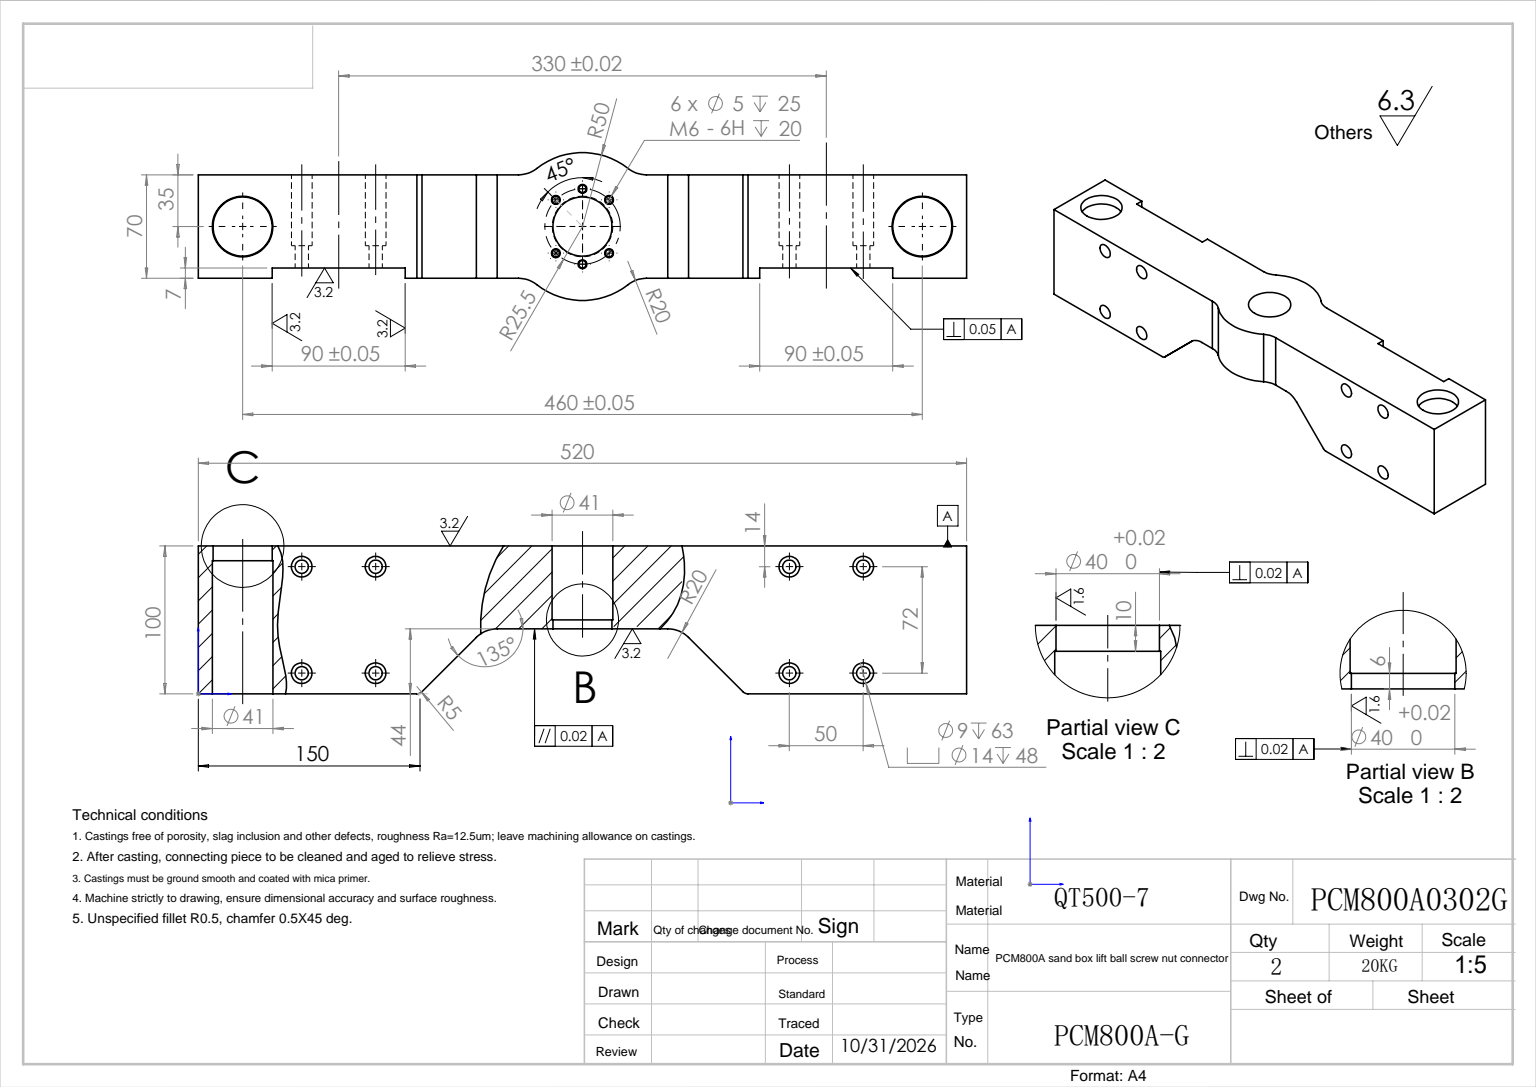
from build123d import *

# Parameters (mm, degrees)
EXTRUDE_1_DEPTH              = 100
CUT_EXTRUDE_1_DEPTH          = 537.306815172
CUT_EXTRUDE_1_DEPTH_BACK     = 537.306815172
SKETCH_3_R                   = 20
CUT_EXTRUDE_2_DEPTH          = 530.868882144
SKETCH_7_R                   = 4.5
CUT_EXTRUDE_4_DEPTH          = 536.242001341
SKETCH_8_R                   = 7
CUT_EXTRUDE_5_DEPTH          = 48
SKETCH_13_R                  = 20
CUT_EXTRUDE_7_DEPTH          = 537.306815172
SKETCH_12_R                  = 1
CUT_EXTRUDE_8_DEPTH          = 10
HOLE_WIZARD_M6_1_D           = 5
HOLE_WIZARD_M6_1_DEPTH       = 25
HOLE_WIZARD_M6_1_CBORE_D     = 6
HOLE_WIZARD_M6_1_CBORE_DEPTH = 20
HOLE_WIZARD_M6_1_TIP         = 1.502151548
SKETCH_18_R                  = 20.5
CUT_EXTRUDE_9_DEPTH          = 90
SKETCH_19_R                  = 20.5
CUT_EXTRUDE_10_DEPTH         = 50
FILLET_1_R                   = 5


with BuildPart() as part:
    # 草图1 → 拉伸1 (new body)
    with BuildSketch(Plane(origin=(0, 0, 0), x_dir=(1, 0, 0), z_dir=(0, 1, 0))):
        with BuildLine():
            Line((0, 70), (0, 0))
            Line((0, 0), (216.698729811, 0))
            ThreePointArc((216.698729811, 0), (223.245266518, -1.10177635), (229.070521293, -4.285714286))
            ThreePointArc((229.070521293, -4.285714286), (260, -15), (290.929478707, -4.285714286))
            ThreePointArc((290.929478707, -4.285714286), (296.754733482, -1.10177635), (303.301270189, 0))
            Line((303.301270189, 0), (520, 0))
            Line((520, 0), (520, 70))
            Line((520, 70), (470, 70))
            Line((470, 70), (470, 63))
            Line((470, 63), (380, 63))
            Line((380, 63), (380, 70))
            Line((380, 70), (303.301270189, 70))
            ThreePointArc((303.301270189, 70), (296.754733482, 71.10177635), (290.929478707, 74.285714286))
            ThreePointArc((290.929478707, 74.285714286), (260, 85), (229.070521293, 74.285714286))
            ThreePointArc((229.070521293, 74.285714286), (223.245266518, 71.10177635), (216.698729811, 70))
            Line((216.698729811, 70), (140, 70))
            Line((140, 70), (140, 63))
            Line((140, 63), (50, 63))
            Line((50, 63), (50, 70))
            Line((50, 70), (0, 70))
        make_face()
    extrude(amount=EXTRUDE_1_DEPTH)

    # 草图2 → 切除-拉伸1 (cut, two sides: drawn at the far end of the back side and taken through both)
    with BuildSketch(Plane.XY.offset(-CUT_EXTRUDE_1_DEPTH_BACK)):
        with BuildLine():
            Line((317.715767105, 43.999711923), (202.284232895, 43.999711923))
            ThreePointArc((202.284232895, 43.999711923), (194.630594492, 42.477315101), (188.142143567, 38.141893843))
            Line((188.142143567, 38.141893843), (150, 0))
            Line((150, 0), (370, 0))
            Line((370, 0), (331.857856433, 38.141893843))
            ThreePointArc((331.857856433, 38.141893843), (325.369405508, 42.477315101), (317.715767105, 43.999711923))
        make_face()
    extrude(amount=CUT_EXTRUDE_1_DEPTH + CUT_EXTRUDE_1_DEPTH_BACK, mode=Mode.SUBTRACT)

    # 草图3 → 切除-拉伸2 (cut, through all)
    with BuildSketch(Plane.XZ.offset(-43.999711923)):
        with Locations((260, -35)):
            Circle(SKETCH_3_R)
    extrude(amount=-CUT_EXTRUDE_2_DEPTH, mode=Mode.SUBTRACT)

    # 草图7 → 切除-拉伸4 (cut, through all)
    with BuildSketch(Plane(origin=(0, 0, -63), x_dir=(-1, 0, 0), z_dir=(0, 0, -1))):
        with Locations((-450, 86)):
            Circle(SKETCH_7_R)
        with Locations((-400, 86)):
            Circle(SKETCH_7_R)
        with Locations((-400, 14)):
            Circle(SKETCH_7_R)
        with Locations((-450, 14)):
            Circle(SKETCH_7_R)
    cut_extrude_4 = extrude(amount=-CUT_EXTRUDE_4_DEPTH, mode=Mode.SUBTRACT)

    # 草图8 → 切除-拉伸5 (cut)
    with BuildSketch(Plane.XY):
        with Locations((400, 86)):
            Circle(SKETCH_8_R)
        with Locations((450, 86)):
            Circle(SKETCH_8_R)
        with Locations((450, 14)):
            Circle(SKETCH_8_R)
        with Locations((400, 14)):
            Circle(SKETCH_8_R)
    cut_extrude_5 = extrude(amount=-CUT_EXTRUDE_5_DEPTH, mode=Mode.SUBTRACT)

    # 镜向2: 切除-拉伸4, 切除-拉伸5 across plane
    add(cut_extrude_4.mirror(Plane(origin=(260, 0, 0), x_dir=(0, 0, 1), z_dir=(1, 0, 0))), mode=Mode.SUBTRACT)
    add(cut_extrude_5.mirror(Plane(origin=(260, 0, 0), x_dir=(0, 0, 1), z_dir=(1, 0, 0))), mode=Mode.SUBTRACT)

    # 草图13 → 切除-拉伸7 (cut, through all)
    with BuildSketch(Plane(origin=(0, 100, 0), x_dir=(1, 0, 0), z_dir=(0, 1, 0))):
        with Locations(Location((30, 35, 0), (0, 0, 270))):
            Circle(SKETCH_13_R)
        with Locations(Location((490, 35, 0), (0, 0, 270))):
            Circle(SKETCH_13_R)
    extrude(amount=-CUT_EXTRUDE_7_DEPTH, mode=Mode.SUBTRACT)

    # 草图12 → 切除-拉伸8 (cut)
    with BuildSketch(Plane.XZ.offset(-43.999711923)):
        with Locations(Location((260, -9.5, 0), (0, 0, 270))):
            Circle(SKETCH_12_R)
        with Locations(Location((241.96877708, -16.96877708, 0), (0, 0, 270))):
            Circle(SKETCH_12_R)
        with Locations(Location((278.03122292, -16.96877708, 0), (0, 0, 270))):
            Circle(SKETCH_12_R)
        with Locations(Location((241.96877708, -53.03122292, 0), (0, 0, 270))):
            Circle(SKETCH_12_R)
        with Locations(Location((260, -60.5, 0), (0, 0, 270))):
            Circle(SKETCH_12_R)
        with Locations(Location((278.03122292, -53.03122292, 0), (0, 0, 270))):
            Circle(SKETCH_12_R)
    extrude(amount=-CUT_EXTRUDE_8_DEPTH, mode=Mode.SUBTRACT)

    # M6 螺纹孔1
    with Locations(Plane.XZ.offset(-43.999711923)):
        with Locations((260, -9.5), (241.96877708, -16.96877708), (278.03122292, -16.96877708), (278.03122292, -53.03122292), (260, -60.5), (241.96877708, -53.03122292)):
            CounterBoreHole(HOLE_WIZARD_M6_1_D / 2, HOLE_WIZARD_M6_1_CBORE_D / 2, HOLE_WIZARD_M6_1_CBORE_DEPTH, depth=HOLE_WIZARD_M6_1_DEPTH)
            with Locations((0, 0, -(HOLE_WIZARD_M6_1_DEPTH + HOLE_WIZARD_M6_1_TIP / 2))):  # 118° drill point
                Cone(0, HOLE_WIZARD_M6_1_D / 2, HOLE_WIZARD_M6_1_TIP, mode=Mode.SUBTRACT)

    # 草图18 → 切除-拉伸9 (cut)
    with BuildSketch(Plane.XZ):
        with Locations(Location((30, -35, 0), (0, 0, 270))):
            Circle(SKETCH_18_R)
        with Locations(Location((490, -35, 0), (0, 0, 270))):
            Circle(SKETCH_18_R)
    extrude(amount=-CUT_EXTRUDE_9_DEPTH, mode=Mode.SUBTRACT)

    # 草图19 → 切除-拉伸10 (cut)
    with BuildSketch(Plane(origin=(0, 100, 0), x_dir=(1, 0, 0), z_dir=(0, 1, 0))):
        with Locations(Location((260, 35, 0), (0, 0, 270))):
            Circle(SKETCH_19_R)
    extrude(amount=-CUT_EXTRUDE_10_DEPTH, mode=Mode.SUBTRACT)

    # 圆角1
    fillet_1_edges = [part.edges().sort_by_distance(p)[0] for p in [
        (150, 0, -35),
        (370, 0, -35),
    ]]
    fillet(fillet_1_edges, radius=FILLET_1_R)


solid = part.part
